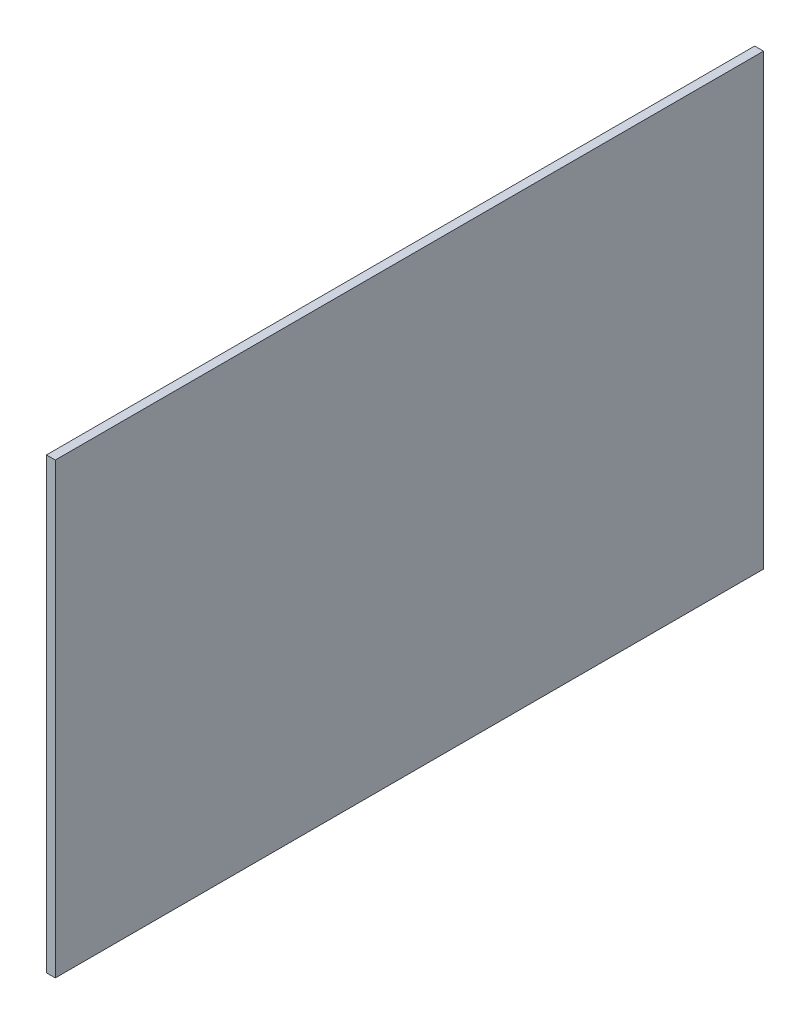
SolidWorks part; units mm, degrees
ref_plane "Front Plane" through (0, 0, 0) normal (0, 0, 1) x (1, 0, 0)
ref_plane "Top Plane" through (0, 0, 0) normal (0, 1, 0) x (1, 0, 0)
ref_plane "Right Plane" through (0, 0, 0) normal (1, 0, 0) x (0, 0, -1)
sketch "Sketch 1" plane through (0, 0, 0) normal (1, 0, 0) x (0, 0, -1)
  line L1 (-60, -38) -> (60, -38)
  line L2 (-60, -38) -> (-60, 38)
  line L3 (-60, 38) -> (60, 38)
  line L4 (60, -38) -> (60, 38)
  line L5 (-60, -38) -> (60, 38) construction
  line L6 (-60, 38) -> (60, -38) construction
  point P0 (0, 0)
  dimension "D1" = 120
  dimension "D2" = 76
extrude "Boss-Extrude 1" add sketch "Sketch 1" along normal blind 1.5
